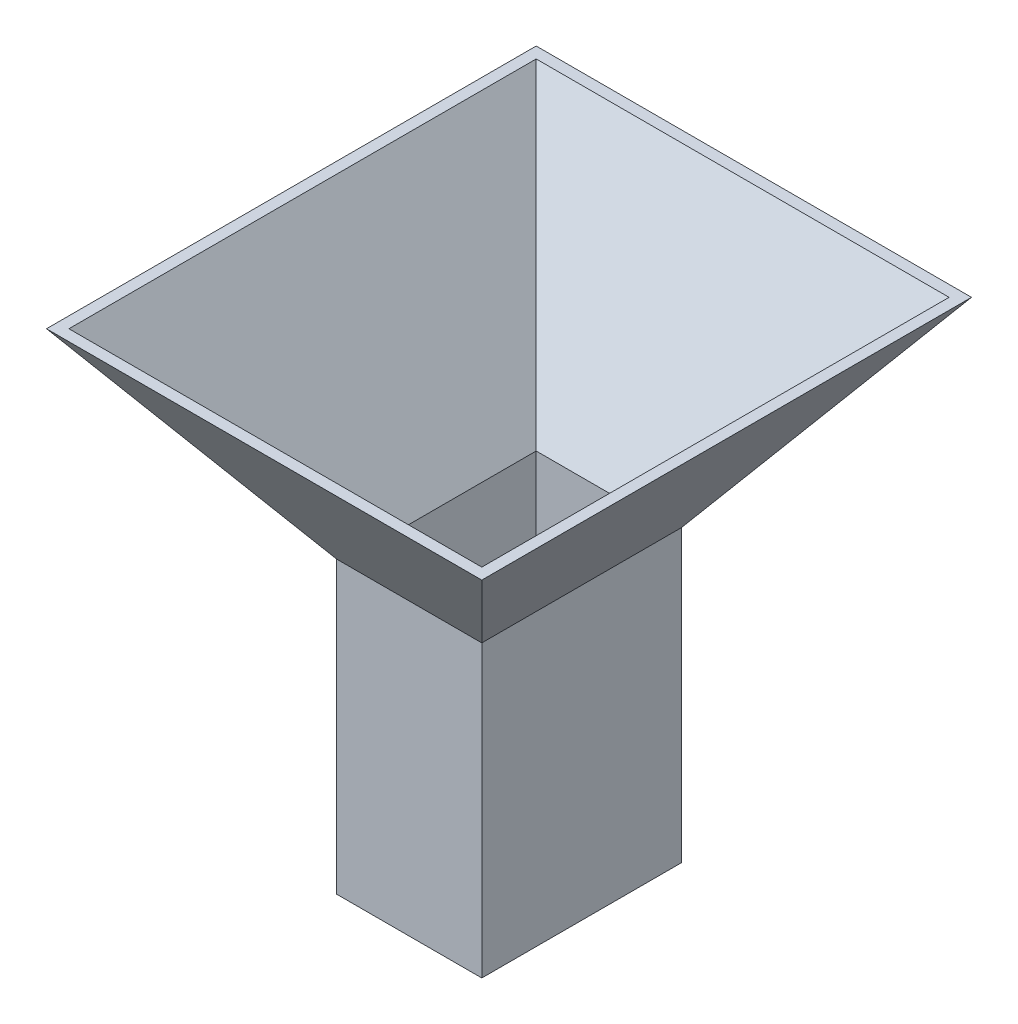
SolidWorks part; units mm, degrees
ref_plane "前视基准面" through (0, 0, 0) normal (0, 0, 1) x (1, 0, 0)
ref_plane "上视基准面" through (0, 0, 0) normal (0, 1, 0) x (1, 0, 0)
ref_plane "右视基准面" through (0, 0, 0) normal (1, 0, 0) x (0, 0, -1)
sketch "草图1" plane through (0, 0, 0) normal (0, 1, 0) x (1, 0, 0)
  line L1 (-40, 55) -> (40, 55)
  line L2 (-40, 55) -> (-40, -55)
  line L3 (-40, -55) -> (40, -55)
  line L4 (40, 55) -> (40, -55)
  line L5 (-40, 55) -> (40, -55) construction
  line L6 (-40, -55) -> (40, 55) construction
  point P0 (0, 0)
  dimension "D1" = 110
  dimension "D2" = 80
extrude "凸台-拉伸1" add sketch "草图1" along normal blind 160
sketch "草图2" plane through (0, 160, 0) normal (0, 1, 0) x (1, 0, 0)
  line L4 (40, -55) -> (40, 55)
  line L5 (40, 55) -> (-40, 55)
  line L6 (-40, 55) -> (-40, -55)
  line L7 (-40, -55) -> (40, -55)
  line L8 (40, -55) -> (40, 55)
  line L9 (40, 55) -> (-40, 55)
  line L10 (-40, 55) -> (-40, -55)
  line L11 (-40, -55) -> (40, -55)
  dimension "D1" = 0
ref_plane "基准面1" through (0, 270, 0) normal (0, 1, 0) x (1, 0, 0)
sketch "草图3" plane through (0, 270, 0) normal (0, 1, 0) x (1, 0, 0)
  line L17 (-120, -135) -> (120, -135)
  line L18 (120, -135) -> (120, 135)
  line L19 (120, 135) -> (-120, 135)
  line L20 (-120, 135) -> (-120, -135)
  line L21 (-120, -135) -> (120, -135)
  line L22 (120, -135) -> (120, 135)
  line L23 (120, 135) -> (-120, 135)
  line L24 (-120, 135) -> (-120, -135)
  dimension "D1" = 80
loft "放样1" add profiles "草图3", "草图2"
sketch "草图4" plane through (-40, 0, 0) normal (-1, 0, 0) x (0, 0, 1)
  line L0 (0, 0) -> (0, 61.6131) construction
  line L1 (100, 0) -> (100, 160)
  line L2 (-100, 0) -> (-100, 160)
  line L3 (-55, 160) -> (55, 160) construction
  line L4 (-55, 0) -> (55, 0) construction
  line L5 (-100, 160) -> (100, 160)
  line L6 (-100, 0) -> (100, 0)
  line L7 (-100, 0) -> (-100, 61.6131) construction
  line L8 (100, 0) -> (100, 61.6131) construction
  dimension "D1" = 100
  dimension "D2" = 100
extrude "凸台-拉伸2" [suppressed] add sketch "草图4" against normal blind 4
shell "抽壳1" thickness 5
sketch "草图5" [suppressed] plane through (-46, 0, 0) normal (1, 0, 0) x (0, 0, -1)
  line L0 (-100, 20) -> (100, 20) construction
  line L1 (-100, 0) -> (-100, 40) construction
  line L2 (100, 40) -> (100, 0) construction
  line L3 (0, 0) -> (0, 73.1022) construction
  circle A0 centre (-90, 20) radius 5
  circle A1 centre (90, 20) radius 5
  dimension "D1" = 10
  dimension "D2" = 180
extrude "切除-拉伸1" [suppressed] cut sketch "草图5" against normal through all
sketch "草图7" plane through (0, 0, -55) normal (0, 0, -1) x (-1, 0, 0)
  line L0 (0, 0) -> (0, 136.8708) construction
  line L1 (-40, 0) -> (40, 0) construction
  line L2 (-31, 45) -> (31, 45)
  line L3 (-31, 45) -> (-31, 65)
  line L4 (-31, 65) -> (31, 65)
  line L5 (31, 45) -> (31, 65)
  line L6 (-31, 45) -> (31, 65) construction
  line L7 (-31, 65) -> (31, 45) construction
  point P3 (0, 55)
  dimension "D1" = 62
  dimension "D2" = 20
  dimension "D3" = 45
extrude "切除-拉伸3" cut sketch "草图7" against normal blind 5
